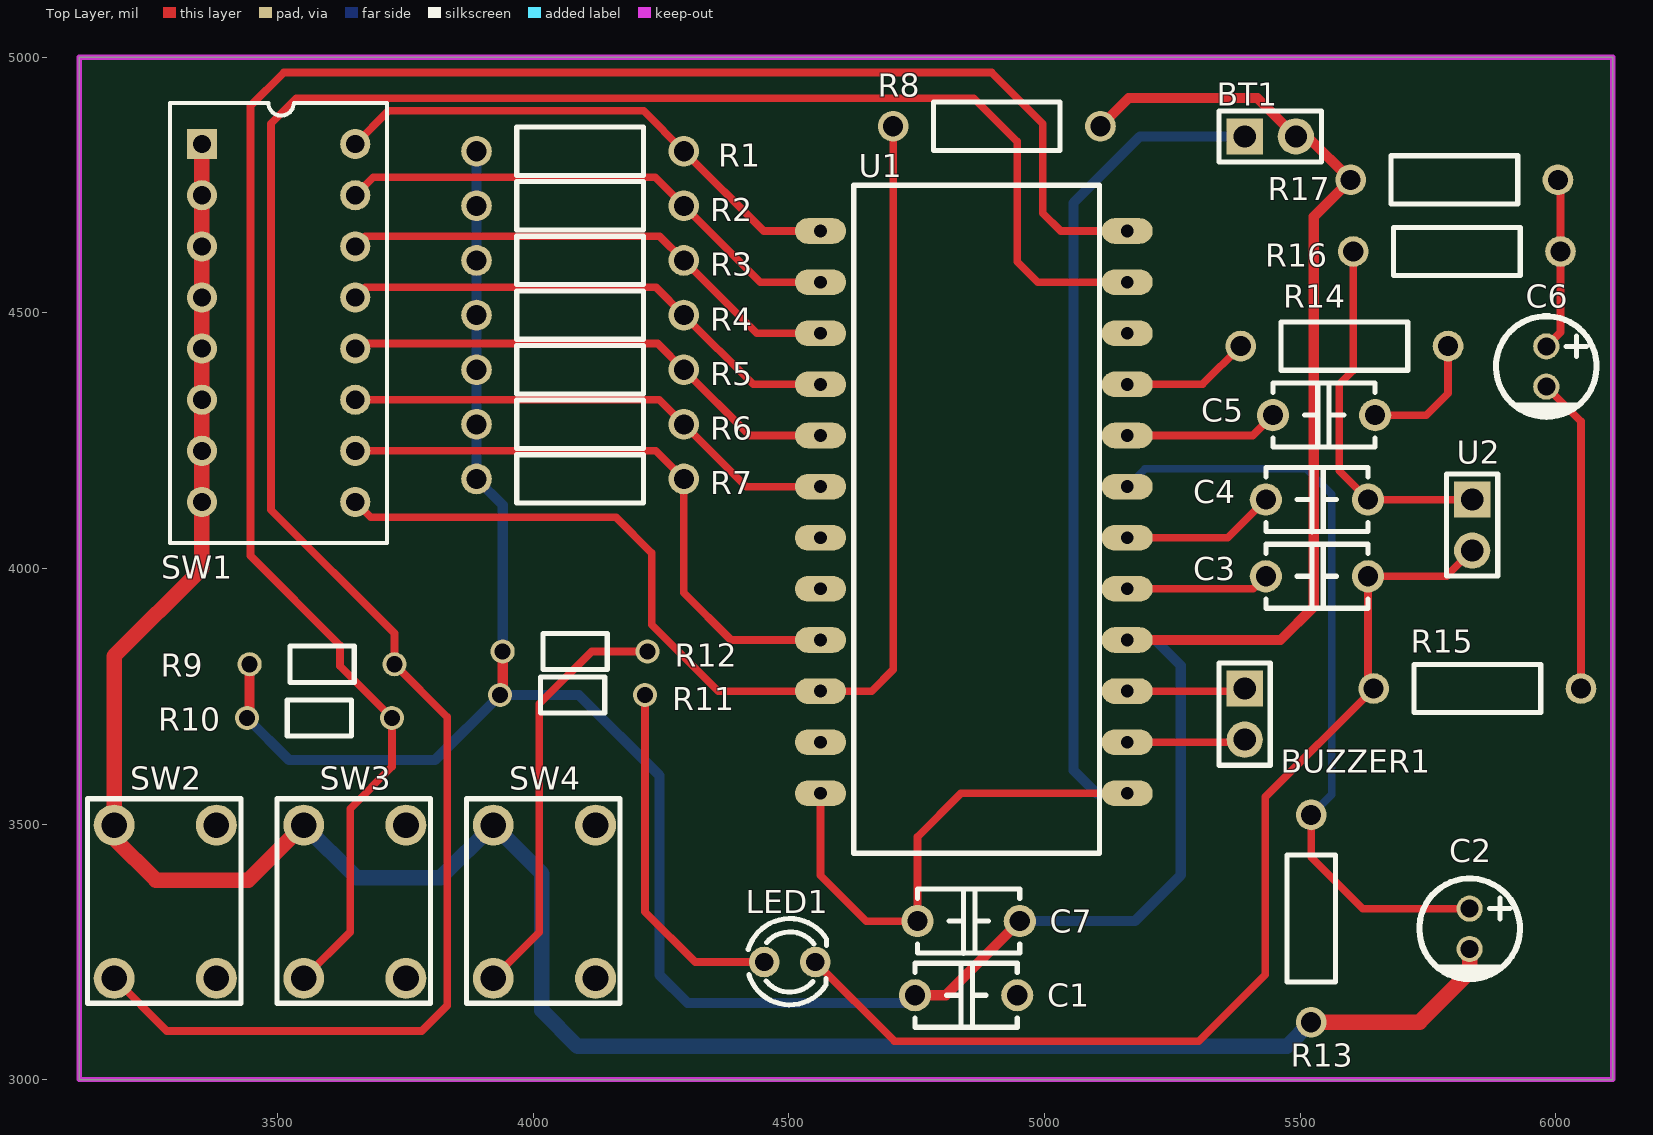
[diagram p0: Top Layer view]
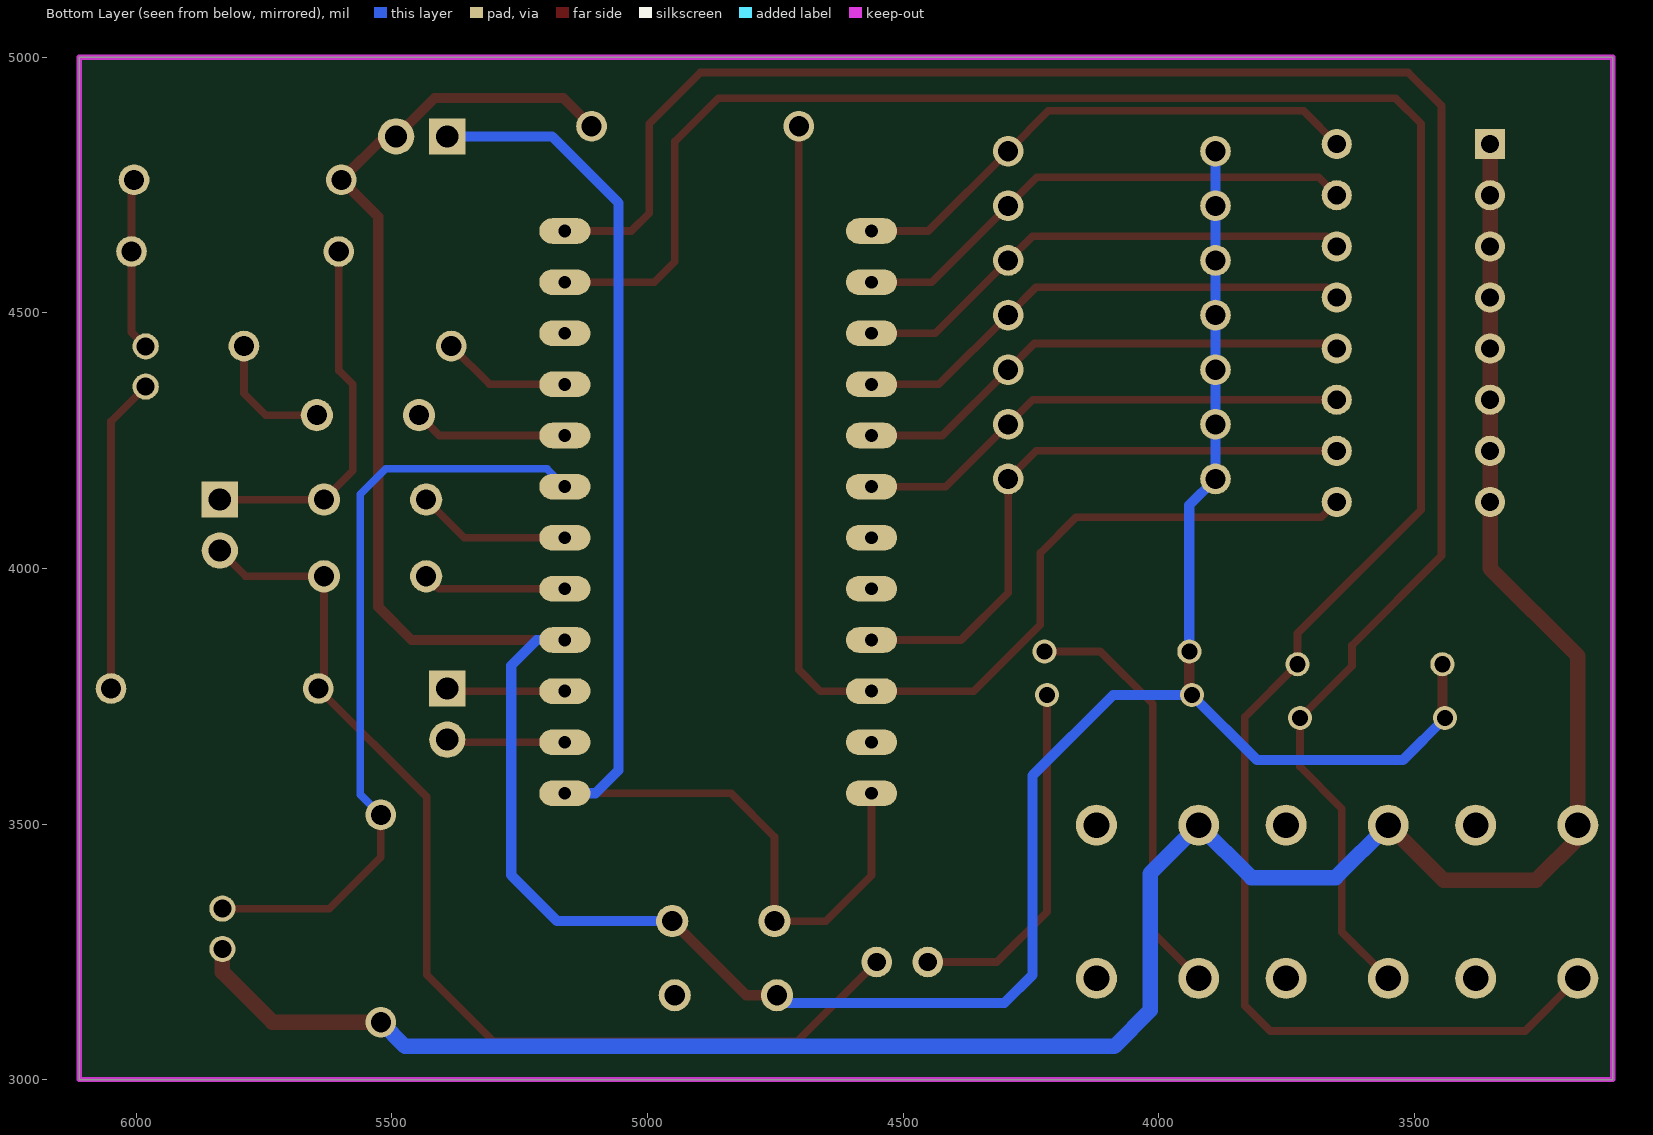
[diagram p1: Bottom Layer view, seen from below]
# Altium PCB MISC51898.pcbdoc
Units mil, origin at the board's own origin, x right, y up, seen from the top; angles counter-clockwise.
Board outline 3000 x 2000 mil, 2 copper layers (Top Layer, Bottom Layer), stack 62.206 mil thick; 33 components, 28 nets, 108 pads, 0 vias.

## Layer stack, top to bottom
Top Solder Mask Layer: solder mask 0.394, Dk 3.3
Top Layer: signal copper 1.379
Dielectric1: surface 59.449, FR4, Dk 4.5
Bottom Layer: signal copper 1.378
Bottom Solder Mask Layer: solder mask 0.394, Dk 3.3

## Board outline
3111.62,5000 3111.62,3000 6111.62,3000 6111.62,5000

## Design rules (kind name [scope] priority, off if disabled: settings)
BoardOutlineClearance copperThickness2oz_1 [All] p2 off: genericclearance=7.99 ignorepadtopadclearanceinfootprint=FALSE except(0: Arc-SplitContinuation Track-SplitContinuation SMDPad-SplitContinuation THPad-SplitContinuation Via-SplitContinuation Fill-SplitContinuation Region-SplitContinuation Poly-SplitContinuation Text-SplitContinuation Hole-SplitContinuation; 5.98: Arc-CutoutEdge SMDPad-CutoutEdge THPad-CutoutEdge Via-CutoutEdge Fill-CutoutEdge Region-CutoutEdge Text-CutoutEdge; 6.93: Hole-OutlineEdge Hole-CutoutEdge; 10: Poly-OutlineEdge Poly-CutoutEdge; 11.81: Arc-OutlineEdge Track-OutlineEdge SMDPad-OutlineEdge THPad-OutlineEdge Via-OutlineEdge Fill-OutlineEdge Region-OutlineEdge Text-OutlineEdge Track-CutoutEdge)
BoardOutlineClearance copperThickness1oz_1 [All] p4: genericclearance=4.02 ignorepadtopadclearanceinfootprint=FALSE except(0: Arc-SplitContinuation Track-SplitContinuation SMDPad-SplitContinuation THPad-SplitContinuation Via-SplitContinuation Fill-SplitContinuation Region-SplitContinuation Poly-SplitContinuation Text-SplitContinuation Hole-SplitContinuation; 6: SMDPad-CutoutEdge THPad-CutoutEdge Via-CutoutEdge Fill-CutoutEdge Region-CutoutEdge Text-CutoutEdge; 6.93: Hole-OutlineEdge Hole-CutoutEdge; 10: Poly-OutlineEdge Poly-CutoutEdge; 11.8: Arc-OutlineEdge Track-OutlineEdge SMDPad-OutlineEdge THPad-OutlineEdge Via-OutlineEdge Fill-OutlineEdge Region-OutlineEdge Text-OutlineEdge; 11.81: Arc-CutoutEdge Track-CutoutEdge)
Clearance copperThickness2oz [All] p1 off: gap=7.99 ignorepadtopadclearanceinfootprint=FALSE except(5.98: SMDPad-Track SMDPad-SMDPad THPad-Track SMDPad-THPad THPad-THPad Track-Via SMDPad-Via THPad-Via Via-Via Fill-Track Region-Track Fill-SMDPad Region-SMDPad Fill-THPad Region-THPad Fill-Via Region-Via Fill-Fill Fill-Region Region-Region Arc-Track Arc-SMDPad Arc-THPad Arc-Via Fill-Arc Region-Arc Arc-Arc Text-Track SMDPad-Text Text-THPad Text-Via Fill-Text Region-Text Arc-Text Text-Text; 6.93: Hole-Track Hole-SMDPad Hole-THPad Hole-Via Fill-Hole Region-Hole Hole-Arc Hole-Text; 10: Poly-Track Poly-SMDPad Poly-THPad Poly-Via Poly-Fill Poly-Region Poly-Poly Poly-Arc Poly-Text Poly-Hole)
Clearance copperThickness1oz [All] p3: gap=4.02 ignorepadtopadclearanceinfootprint=FALSE except(5.98: SMDPad-Track SMDPad-SMDPad THPad-Track SMDPad-THPad THPad-THPad Track-Via SMDPad-Via THPad-Via Via-Via Fill-Track Region-Track Fill-SMDPad Region-SMDPad Fill-THPad Region-THPad Fill-Via Region-Via Fill-Fill Fill-Region Region-Region; 6: Arc-Track Arc-SMDPad Arc-THPad Arc-Via Fill-Arc Region-Arc Arc-Arc Text-Track SMDPad-Text Text-THPad Text-Via Fill-Text Region-Text Arc-Text Text-Text; 6.93: Hole-Track Hole-SMDPad Hole-THPad Hole-Via Fill-Hole Region-Hole Hole-Arc Hole-Text; 10: Poly-Track Poly-SMDPad Poly-THPad Poly-Via Poly-Fill Poly-Region Poly-Poly Poly-Arc Poly-Text Poly-Hole)
Creepage creepage [All] p1: checkdistance=0 ignoreinternallayers=TRUE applytopolygonpour=TRUE
DiffPairsRouting differentialPair [All] p1: maxlimit=6 minlimit=6 mostfreqgap=6 toplayer_minwidth=5 toplayer_prefwidth=10 toplayer_maxwidth=100 toplayer_mingap=6 toplayer_prefgap=6 toplayer_maxgap=6 bottomlayer_minwidth=5 bottomlayer_prefwidth=10 bottomlayer_maxwidth=100 bottomlayer_mingap=6 bottomlayer_prefgap=6 bottomlayer_maxgap=6 maxuncoupledlength=10
HoleToHoleClearance otherClearance [All] p1: gap=11.81 allowstackedmicrovias=TRUE
Length netLength [All] p1: minlimit=0 maxlimit=0
MatchedLengths netLengthTolerance [All] p1: tolerance=1000
PasteMaskExpansion pasteMaskExpansion [All] p1: expansion=0
PlaneConnect innerPlane [All] p1: planeconnectstyle=Relief reliefexpansion=20 reliefentries=4 reliefconductorwidth=10 reliefairgap=10
PolygonConnect copperRegion [All] p1: connectstyle=Relief reliefconductorwidth=10 reliefentries=4 polygonreliefangle="90 Angle" airgapwidth=10 via.connectstyle=Relief via.reliefconductorwidth=10 via.reliefentries=4 via.polygonreliefangle="90 Angle" via.airgapwidth=10
RoutingVias viaSize [All] p1: holewidth=12.01 width=24.02 viastyle="Through Hole" minholewidth=11.81 minwidth=19.68 maxholewidth=248.03 maxwidth=393.7
SolderMaskExpansion solderMaskExpansion [IsVia] p1: expansion=-1000 istentingtop=TRUE
SolderMaskExpansion solderMaskExpansion [All] p2: expansion=2 istentingtop=FALSE
Width copperThickness2oz_2 [All] p1 off: maxlimit=100 minlimit=8 preferedwidth=10
Width copperThickness1oz_2 [All] p2: maxlimit=100 minlimit=5 preferedwidth=10

## Components (designator, comment, footprint, x,y, rotation, side; value= is the part's Value field where it differs from the comment)
BT1 "" HDR-TH_2P-P2.54-V-M-1 5441.62,4845 r0 top
BUZZER1 "SPEAKER" HDR-TH_2P-P2.54-V-M-1 5391.62,3715 r270 top
C1 "0.0uF" CAP-TH_L5.1-W3.2-P5.08-D0.50 4846.62,3165 r0 top
C2 "4.7uF" CAP-TH_BD5.0-P2.00-D0.8-FD-10UF50VC110GL 5831.62,3295 r270 top
C3 "0.1uF" CAP-TH_L5.1-W3.2-P5.08-D0.50 5532.89,3984.58 r0 top
C4 "0.1uF" CAP-TH_L5.1-W3.2-P5.08-D0.50 5532.89,4134.58 r0 top
C5 "0.1uF" CAP-TH_L5.1-W3.2-P5.08-D0.50 5546.81,4299.8 r180 top
C6 "220uF" CAP-TH_BD5.0-P2.00-D0.8-FD-10UF50VC110GL 5981.62,4395 r270 top
C7 "0.1uF" CAP-TH_L5.1-W3.2-P5.08-D0.50 4851.62,3310 r0 top
LED1 "" LED_TH-3mm 4501.62,3230 r0 top
R1 "10kΩ" Res_1/4W 4091.62,4816.18 r180 top
R2 "10kΩ" Res_1/4W 4091.62,4709.32 r180 top
R3 "10kΩ" Res_1/4W 4091.62,4602.45 r180 top
R4 "10kΩ" Res_1/4W 4091.62,4495.59 r180 top
R5 "10kΩ" Res_1/4W 4091.62,4388.73 r180 top
R6 "10kΩ" Res_1/4W 4091.62,4281.86 r180 top
R7 "10kΩ" Res_1/4W 4091.62,4175 r180 top
R8 "10kΩ" Res_1/4W 4906.62,4865 r0 top
R9 "100kΩ" Res_1/8W 3586.62,3810 r0 top
R10 "100kΩ" Res_1/8W 3581.62,3705 r0 top
R11 "5.1kΩ" Res_1/8W 4076.62,3750 r0 top
R12 "100kΩ" Res_1/8W 4081.62,3835 r0 top
R13 "470kΩ" Res_1/4W 5521.62,3315 r90 top
R14 "5.1kΩ" Res_1/4W 5586.62,4435 r180 top
R15 "10kΩ" Res_1/4W 5846.62,3765 r0 top
R16 "10kΩ" Res_1/4W 5806.62,4620 r0 top
R17 "1kΩ" Res_1/4W 5801.62,4760 r180 top
SW1 "SW-DIP8" SW-DIP8 3501.62,4420 r90 top
SW2 "" SW-TH_4P-L6.0-W6.0-P4.50-LS6.5 3180,3497.89 r0 top
SW3 "" SW-TH_4P-L6.0-W6.0-P4.50-LS6.5 3550.81,3497.89 r0 top
SW4 "" SW-TH_4P-L6.0-W6.0-P4.50-LS6.5 3921.62,3497.89 r0 top
U1 "" DIP-24_L30.4-W12.7-P2.54-LS10.1-BL 4561.62,4160 r270 top
U2 "" HDR-TH_2P-P2.54-V-M-1 5836.62,4085 r270 top

## Footprints (in the part's own frame and the unit in brackets; to place one, negate y for a bottom-side part, rotate by r counter-clockwise, add the part's x,y. Pads: shape width x height; smd on the part's side, far side on the other; paste and mask are expansions set on the pad)
CAP-TH_BD5.0-P2.00-D0.8-FD-10UF50VC110GL [mm]
  round 1.3 hole 0.9 paste+0 mask+0.051: 1(-1,0) 2(1,0)
  silkscreen extent -2.5,-2.5 2.5,2.5
CAP-TH_L5.1-W3.2-P5.08-D0.50 [mm]
  round 1.6 hole 1 paste+0 mask+0.05: 1(-2.54,0) 2(2.54,0)
  silkscreen extent -2.54,-1.6 2.54,1.59
DIP-24_L30.4-W12.7-P2.54-LS10.1-BL [mil]
  oval 50x100 hole 25 paste+0 mask+1.97: 1(-500,0) 2(-400,0) 3(-300,0) 4(-200,0) 5(-100,0) 6(0,0) 7(100,0) 8(200,0) 9(300,0) 10(400,0) 11(500,0) 12(600,0) 13(600,600) 14(500,600) 15(400,600) 16(300,600) 17(200,600) 18(100,600) 19(0,600) 20(-100,600) 21(-200,600) 22(-300,600) 23(-400,600) 24(-500,600)
  silkscreen extent -590,65 717,546
HDR-TH_2P-P2.54-V-M-1 [mm]
  rect 1.8x1.8 hole 1.1: 1(-1.27,0)
  round 1.8 hole 1.1: 2(1.27,0)
  silkscreen extent -2.54,-1.27 2.54,1.27
LED_TH-3mm [mil]
  round 60 hole 36 paste+0 mask+2: 1(-50,0) 2(50,0)
  silkscreen extent -81,-84 72,85
Res_1/4W [mil]
  round 60 hole 39.37 paste+0 mask+2: 1(-202.76,0) 2(202.76,0)
  silkscreen extent -124,-47 124,47
Res_1/8W [mil]
  round 47.2 hole 31.5 paste+0 mask+2: 1(-141.7,2.48) 2(141.7,2.48)
  silkscreen extent -63,-33 63,38
SW-DIP8 [mm]
  rect 1.5x1.5 hole 0.9: 1(10.414,3.81)
  round 1.5 hole 0.9: 2(7.874,3.81) 3(5.334,3.81) 4(2.794,3.81) 5(0.254,3.81) 6(-2.286,3.81) 7(-4.826,3.81) 8(-7.366,3.81) 9(-7.366,-3.81) 10(-4.826,-3.81) 11(-2.286,-3.81) 12(0.254,-3.81) 13(2.794,-3.81) 14(5.334,-3.81) 15(7.874,-3.81) 16(10.414,-3.81)
  silkscreen extent -9.42,-5.39 12.46,5.4
SW-TH_4P-L6.0-W6.0-P4.50-LS6.5 [mil]
  round 80 hole 50: 1(0,0) 2(200,0) 3(0,-299.96) 4(200,-299.96)
  silkscreen extent -52,-349 248,51

## Nets (pads, with @x,y where several pads share a name; then routed paths per layer and width w, separated by ;. In a path a pad name is that pad's centre, name@x,y a point inside that pad or via, vN(x,y) a via of type N, cw(c..) or ccw(c..) an arc to the next point about the centre after c; other vN are vias at no path point)
$1N1: R2.1 SW1.15 U1.2 | length 1009.4
  Top Layer w15: SW1.15 3686.62,4765 4238.69,4765 R2.1 4443.69,4560 U1.2
$1N2: R1.1 SW1.16 U1.1 | length 1034.3
  Top Layer w15: SW1.16 3716.62,4895 4215.56,4895 R1.1 4450.56,4660 U1.1
$1N3: R3.1 SW1.14 U1.3 | length 997
  Top Layer w15: SW1.14 3671.62,4650 4246.83,4650 R3.1 4436.83,4460 U1.3
$1N4: R4.1 SW1.13 U1.4 | length 997
  Top Layer w15: SW1.13 3671.62,4550 4239.97,4550 R4.1 4429.97,4360 U1.4
$1N5: R5.1 SW1.12 U1.5 | length 988.7
  Top Layer w15: SW1.12 3661.62,4440 4243.1,4440 R5.1 4423.1,4260 U1.5
$1N6: R6.1 SW1.11 U1.6 | length 980.4
  Top Layer w15: SW1.11 4246.24,4330 R6.1 4416.24,4160 U1.6
$1N7: R7.1 SW1.10 U1.9 | length 1193.7
  Top Layer w15: SW1.10 4239.38,4230 R7.1 4294.38,3952.24 4386.62,3860 U1.9
$1N8: R8.1 SW1.9 U1.10 | length 2367.8
  Top Layer w15: SW1.9 3681.62,4100 4161.62,4100 4231.62,4030 4231.62,3890 4361.62,3760 U1.10 4661.62,3760 4703.86,3802.24 R8.1
$1N11: R9.2 SW2.3 U1.23 | length 4565.4
  Top Layer w15: SW2.3 3282.93,3095 3781.62,3095 3831.62,3145 3831.62,3709.18 R9.2 3728.32,3873.3 3486.62,4115 3486.62,4870 3536.62,4920 4861.62,4920 4946.62,4835 4946.62,4600 4986.62,4560 U1.23
$1N12: R10.2 SW3.3 U1.24 | length 3866
  Top Layer w15: SW3.3 3641.62,3288.74 3641.62,3530 3723.32,3611.7 R10.2 3621.62,3809.18 3621.62,3850 3446.62,4025 3446.62,4905 3511.62,4970 4896.62,4970 4996.62,4870 4996.62,4695 5031.62,4660 U1.24
$1N13: C1.2
$1N14: LED1.1 R11.2 | length 698.2
  Top Layer w15: R11.2 4218.32,3328.3 4316.62,3230 LED1.1
$1N15: C3.2 LED1.2 R15.1 U2.2 | length 2094.7
  Top Layer w15: LED1.2 4706.62,3075 5301.62,3075 5431.62,3205 5431.62,3552.76 R15.1 5632.89,3775.97 C3.2 5786.2,3984.58 U2.2
$1N17: R12.2 SW4.3 | length 828.5
  Top Layer w15: SW4.3 4011.62,3287.93 4011.62,3735 4114.09,3837.48 R12.2
$1N20: C2.1 R13.2 U1.19 | length 1513.5
  Top Layer w15: R13.2 5521.62,3435 5622.25,3334.37 C2.1
  Bottom Layer w15: U1.19 5196.62,4195 5511.62,4195 5561.62,4145 5561.62,3557.76 R13.2
$1N22: C3.1 U1.17 | length 281.5
  Top Layer w15: U1.17 5408.31,3960 C3.1
$1N23: C4.1 U1.18 | length 302.2
  Top Layer w15: U1.18 5358.31,4060 C4.1
$1N24: C4.2 R16.1 U2.1 | length 723.9
  Top Layer w15: R16.1 5603.86,4387.24 5576.62,4360 5576.62,4190.86 C4.2 5836.2,4134.58 U2.1
$1N25: BUZZER1.2 U1.14 | length 232.1
  Top Layer w15: U1.14 5386.62,3660 BUZZER1.2
$1N26: BUZZER1.1 U1.15 | length 232.1
  Top Layer w15: U1.15 5386.62,3760 BUZZER1.1
$1N27: C5.1 R14.1 | length 252.6
  Top Layer w15: C5.1 5746.42,4299.8 5789.38,4342.76 R14.1
$1N28: R14.2 U1.21 | length 253.3
  Top Layer w15: U1.21 5308.86,4360 R14.2
$1N29: C5.2 U1.20 | length 301.7
  Top Layer w15: U1.20 5407.01,4260 C5.2
$1N30: C6.2 R15.2 | length 618.7
  Top Layer w15: C6.2 6049.38,4287.87 R15.2
$1N31: C6.1 R16.2 R17.1 | length 339.2
  Top Layer w15: C6.1 6009.38,4462.13 R16.2 6009.38,4755 R17.1
$1N33: BT1.1 C7.1 U1.12 U1.13 | length 2620
  Top Layer w15: U1.12 4561.62,3400 4651.62,3310 C7.1 4751.62,3475 4836.62,3560 U1.13
  Bottom Layer w20: U1.13 5101.62,3560 5056.62,3605 5056.62,4715 5186.62,4845 BT1.1
GND: C2.2 R13.1 SW1.1 SW1.2 SW1.3 SW1.4 SW1.5 SW1.6 SW1.7 SW1.8 SW2.1 SW3.1 SW4.1 | length 4686.7
  Top Layer w30: SW1.1 SW1.2 SW1.3 SW1.4 SW1.5 SW1.6 SW1.7 SW1.8 3351.62,4000 3180,3828.38 SW2.1 3180,3471.62 3261.62,3390 3442.92,3390 SW3.1 ; R13.1 5733.86,3112.24 5831.62,3210 C2.2
  Bottom Layer w30: SW3.1 3653.7,3395 3818.73,3395 SW4.1 4016.62,3402.89 4016.62,3135 4086.62,3065 5474.38,3065 R13.1
VCC: BT1.2 C1.1 C7.2 R1.2 R2.2 R3.2 R4.2 R5.2 R6.2 R7.2 R8.2 R9.1 R10.1 R11.1 R12.1 R17.2 U1.16 | length 6060.3
  Top Layer w20: R10.1 3444.92,3712.48 R9.1 ; R11.1 3939.92,3757.48 R12.1 ; C1.1 4806.62,3165 C7.2 ; R8.2 5164.38,4920 5416.62,4920 BT1.2 5513.86,4845 R17.2 5526.62,4687.76 5526.62,3925 5461.62,3860 U1.16
  Bottom Layer w20: R10.1 3522.39,3625 3807.44,3625 R11.1 4089.14,3752.48 4246.62,3595 4246.62,3205 4301.62,3150 4731.62,3150 C1.1 ; R1.2 R2.2 R3.2 R4.2 R5.2 R6.2 R7.2 3939.92,4123.94 R12.1 ; C7.2 5176.62,3310 5266.62,3400 5266.62,3810 5216.62,3860 U1.16
pads on no net: SW2.2 SW2.4 SW3.2 SW3.4 SW4.2 SW4.4 U1.7 U1.8 U1.11 U1.22

## Keep-outs
Board Outline Layer:
  the board outline again, w10